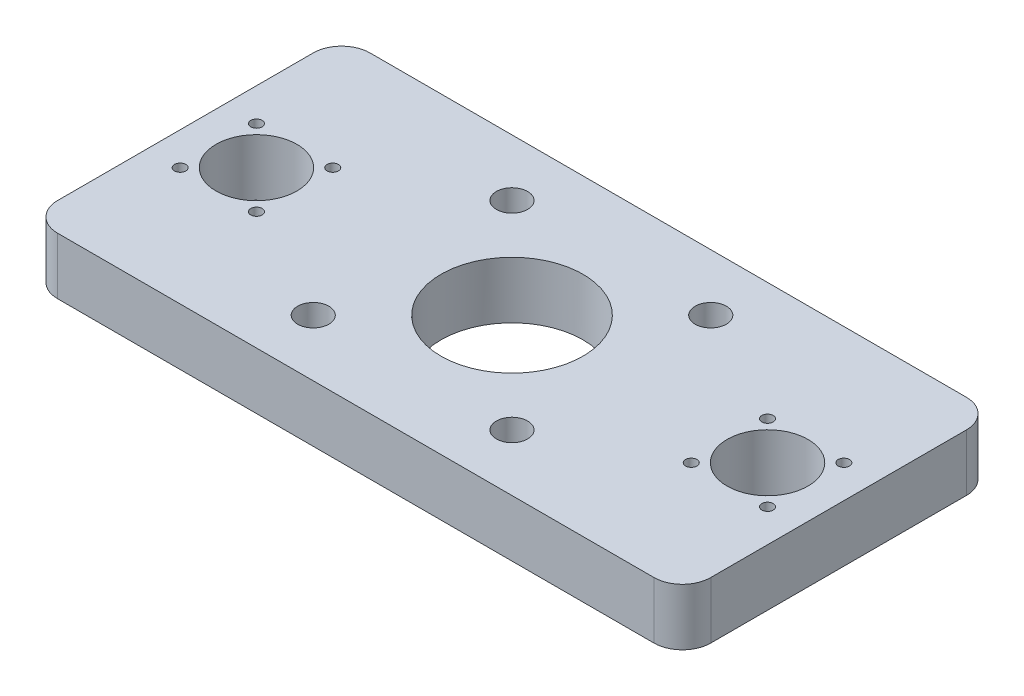
from build123d import *

# Parameters (mm, degrees)
SKETCH1_W              = 230
SKETCH1_H              = 110
BOSS_EXTRUDE1_DEPTH    = 20
SKETCH2_R              = 14.25
CUT_EXTRUDE2_DEPTH     = 256.734237051
SKETCH3_R              = 2
CUT_EXTRUDE3_DEPTH     = 256.734237051
LPATTERN1_COUNT        = 2
LPATTERN1_PITCH        = 180
FILLET1_R              = 10
SKETCH4_R              = 25
SKETCH4_R_2            = 5.5
CUT_EXTRUDE4_DEPTH     = 100
M12_TAPPED_HOLE2_D     = 10.2
M12_TAPPED_HOLE2_DEPTH = 20
M12_TAPPED_HOLE2_TIP   = 3.064389157


with BuildPart() as part:
    # Sketch1 → Boss-Extrude1 (new body)
    with BuildSketch(Plane(origin=(0, 0, 0), x_dir=(1, 0, 0), z_dir=(0, 1, 0))):
        with Locations((115, 55)):
            Rectangle(SKETCH1_W, SKETCH1_H)
    extrude(amount=BOSS_EXTRUDE1_DEPTH)

    # Sketch2 → Cut-Extrude2 (cut, through all)
    with BuildSketch(Plane(origin=(0, 20, 0), x_dir=(1, 0, 0), z_dir=(0, 1, 0))):
        with Locations(Location((25, 55, 0), (0, 0, 270))):
            Circle(SKETCH2_R)
        with Locations(Location((205, 55, 0), (0, 0, 270))):
            Circle(SKETCH2_R)
    extrude(amount=-CUT_EXTRUDE2_DEPTH, mode=Mode.SUBTRACT)

    # Sketch3 → Cut-Extrude3 (cut, through all)
    with BuildSketch(Plane(origin=(0, 20, 0), x_dir=(1, 0, 0), z_dir=(0, 1, 0))):
        with Locations(Location((11.564971157, 68.435028843, 0), (0, 0, 270))):
            Circle(SKETCH3_R)
        with Locations(Location((38.435028843, 68.435028843, 0), (0, 0, 270))):
            Circle(SKETCH3_R)
        with Locations(Location((38.435028843, 41.564971157, 0), (0, 0, 270))):
            Circle(SKETCH3_R)
        with Locations(Location((11.564971157, 41.564971157, 0), (0, 0, 270))):
            Circle(SKETCH3_R)
    cut_extrude3 = extrude(amount=-CUT_EXTRUDE3_DEPTH, mode=Mode.SUBTRACT)

    # LPattern1: Cut-Extrude3 ×2
    with Locations(*[(i * LPATTERN1_PITCH, 0, 0) for i in range(1, LPATTERN1_COUNT)]):
        add(cut_extrude3, mode=Mode.SUBTRACT)

    # Fillet1
    fillet1_edges = [part.edges().sort_by_distance(p)[0] for p in [
        (0, 10, 0),
        (0, 10, -110),
        (230, 10, -110),
        (230, 10, 0),
    ]]
    fillet(fillet1_edges, radius=FILLET1_R)

    # Sketch4 → Cut-Extrude4 (cut)
    with BuildSketch(Plane(origin=(0, 20, 0), x_dir=(1, 0, 0), z_dir=(0, 1, 0))):
        with Locations(Location((115, 55, 0), (0, 0, 270))):
            Circle(SKETCH4_R)
        with Locations(Location((150, 90, 0), (0, 0, 270))):
            Circle(SKETCH4_R_2)
        with Locations(Location((150, 20, 0), (0, 0, 270))):
            Circle(SKETCH4_R_2)
        with Locations(Location((80, 20, 0), (0, 0, 270))):
            Circle(SKETCH4_R_2)
        with Locations(Location((80, 90, 0), (0, 0, 270))):
            Circle(SKETCH4_R_2)
    extrude(amount=-CUT_EXTRUDE4_DEPTH, mode=Mode.SUBTRACT)

    # M12 Tapped Hole2
    with Locations(Plane(origin=(0, 0, -110), x_dir=(-1, 0, 0), z_dir=(0, 0, -1))):
        with Locations((-200, 10), (-115, 10), (-30, 10)):
            Hole(M12_TAPPED_HOLE2_D / 2, depth=M12_TAPPED_HOLE2_DEPTH)
            with Locations((0, 0, -(M12_TAPPED_HOLE2_DEPTH + M12_TAPPED_HOLE2_TIP / 2))):  # 118° drill point
                Cone(0, M12_TAPPED_HOLE2_D / 2, M12_TAPPED_HOLE2_TIP, mode=Mode.SUBTRACT)


solid = part.part
